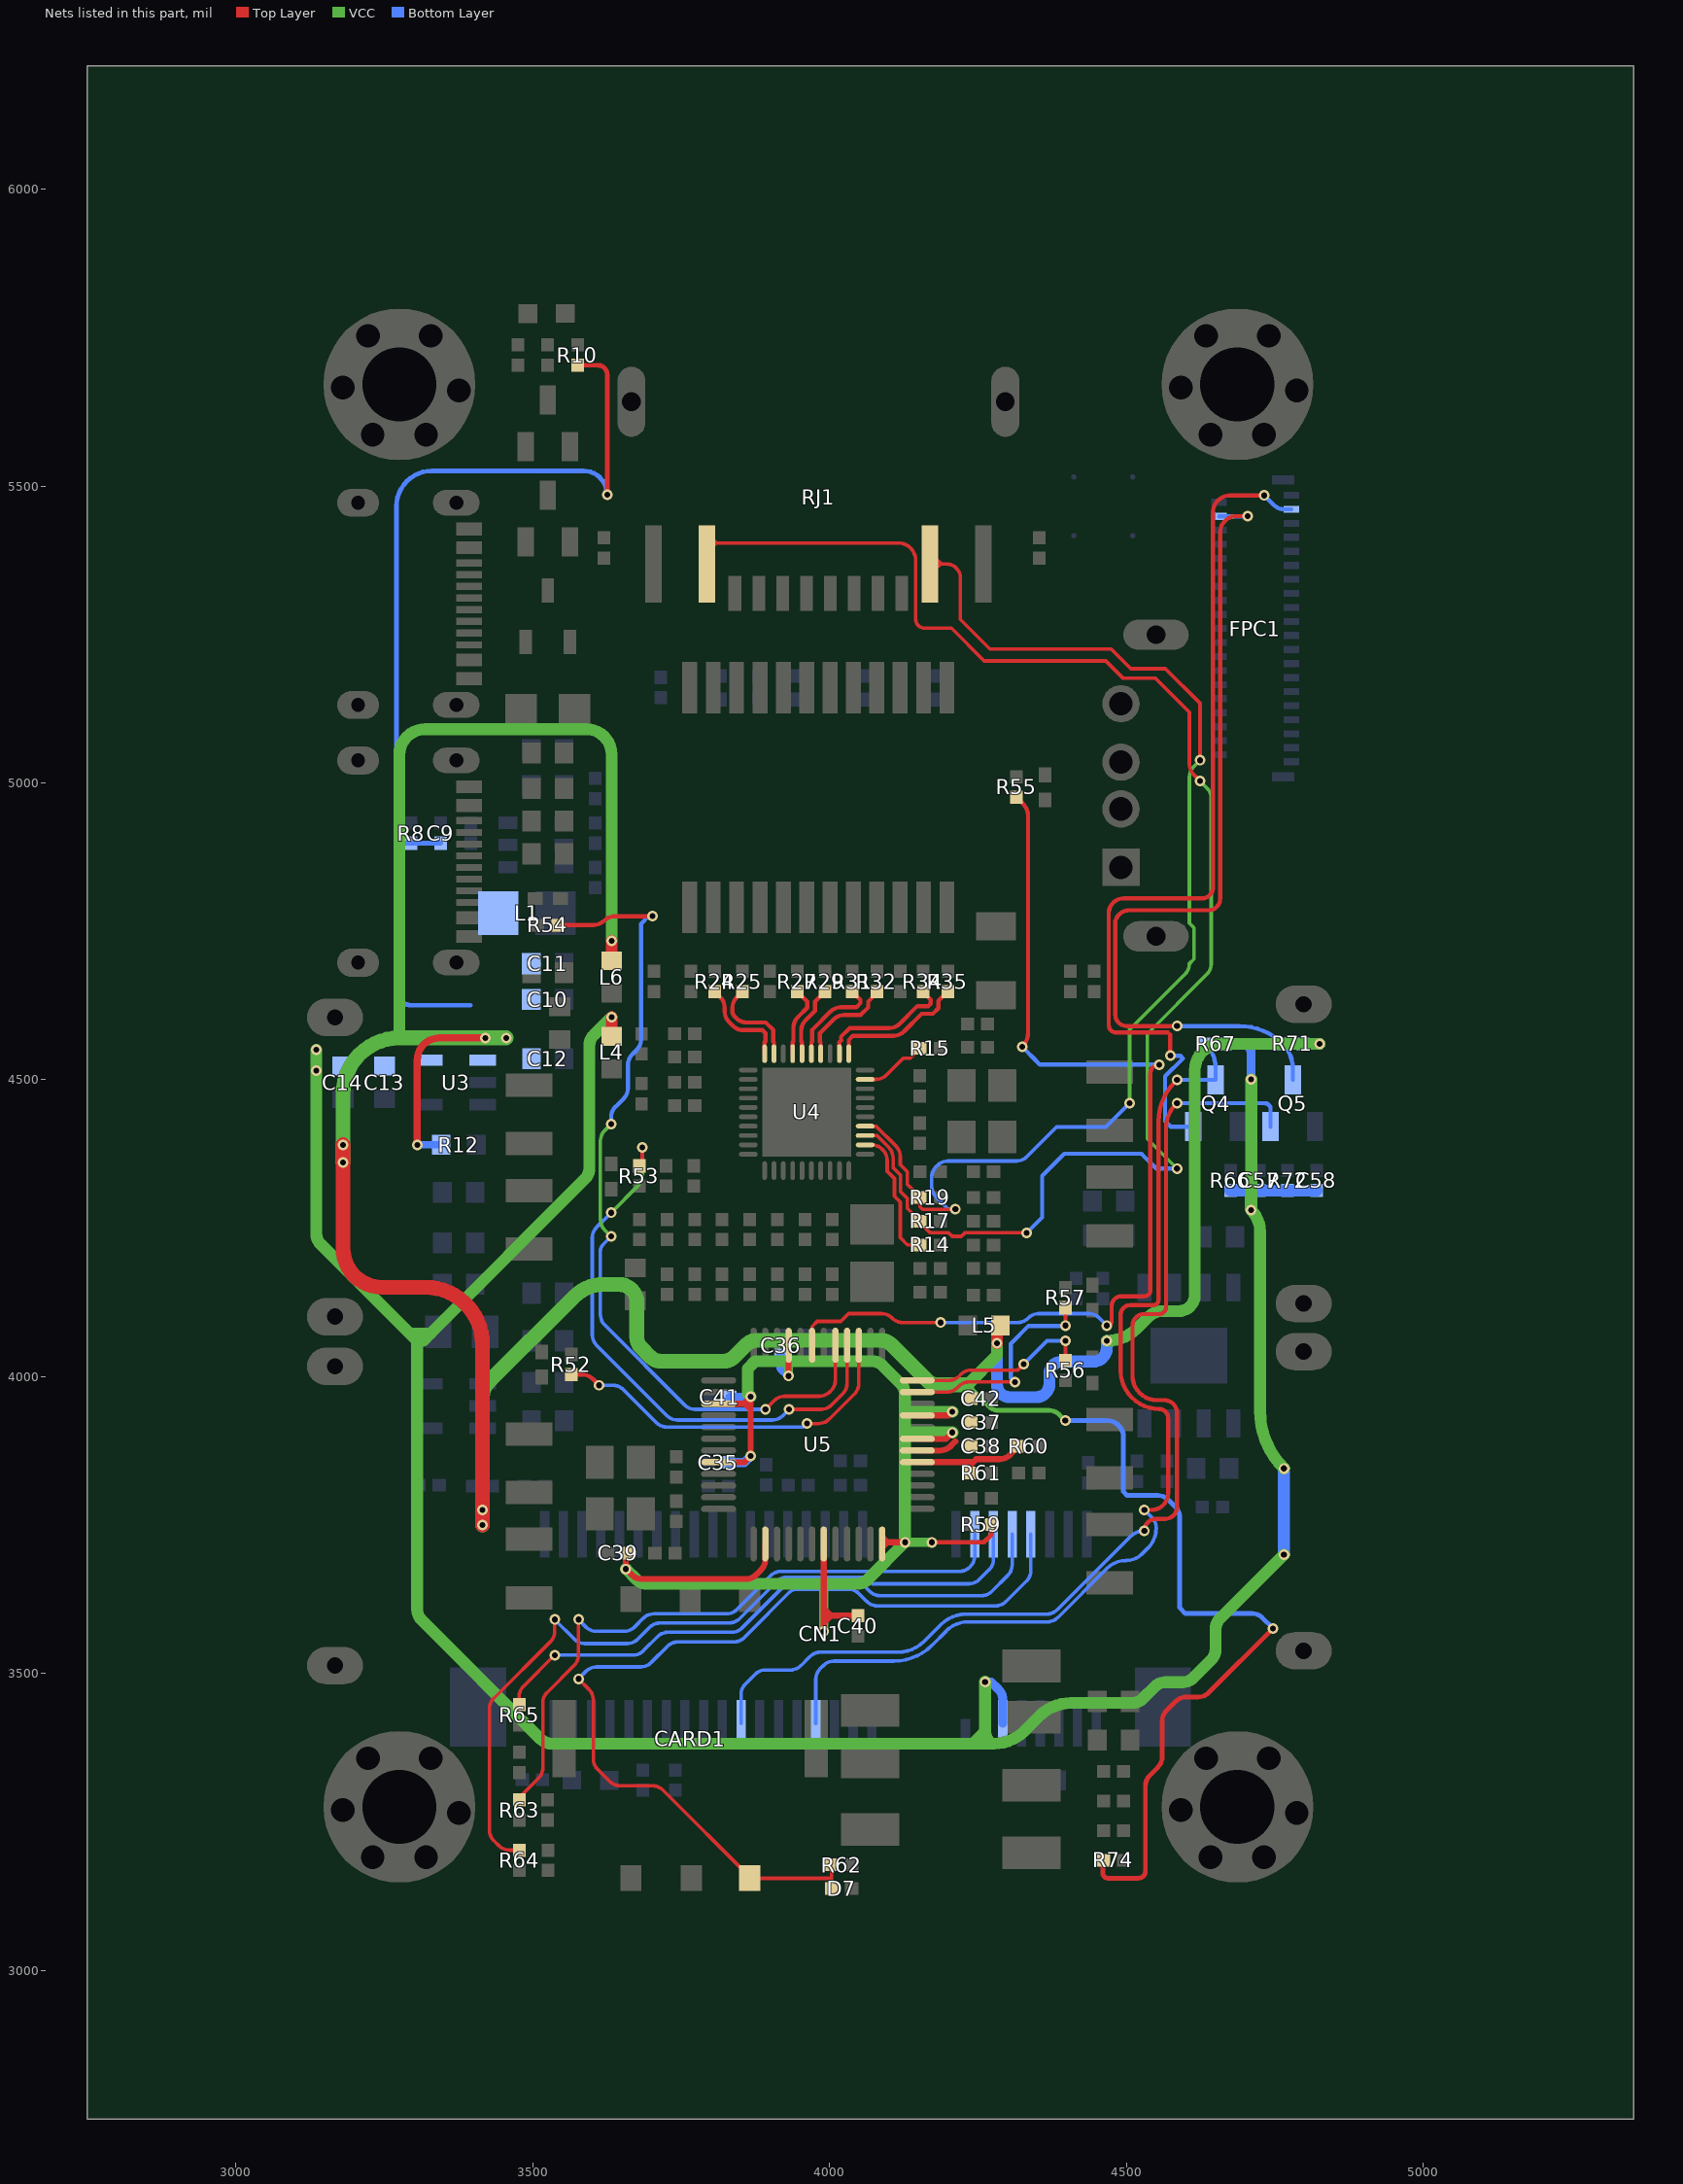
[diagram p0: the nets of this part, all layers, seen from the top]
# Altium PCB MISC84334.PcbDoc (part 7 of 8)
Units mil, origin at the board's own origin, x right, y up, seen from the top; angles counter-clockwise.
Board outline 2605.13 x 3457.4 mil, 4 copper layers (Top Layer, GND, VCC, Bottom Layer), stack 62.447 mil thick; 209 components, 149 nets, 735 pads, 529 vias.

## Via types
v1: diameter 18, hole 10, Top Layer to Bottom Layer, 529 vias

## Nets (pads, with @x,y where several pads share a name; then routed paths per layer and width w, separated by ;. In a path a pad name is that pad's centre, name@x,y a point inside that pad or via, vN(x,y) a via of type N, cw(c..) or ccw(c..) an arc to the next point about the centre after c; other vN are vias at no path point) (continued)
LED1: R52.2 U5.3 | length 616.2
  Top Layer w6: v1(3962.29,3921.19) 3981.94,3921.19 ccw(c3981.94,3946.19) 3999.61,3928.51 4042.17,3971.07 ccw(c4024.49,3988.75) 4049.49,3988.75 U5.3@4049.49,4052.91
  Top Layer w7: R52.2@3565.22,4003.55 3583.98,4003.55 cw(c3583.98,3978.55) 3601.65,3996.23 v1(3612.29,3985.59)
  Bottom Layer w6: v1(3612.29,3985.59) 3635.24,3985.59 cw(c3635.24,3960.59) 3652.91,3978.27 3708.67,3922.51 ccw(c3726.35,3940.19) 3726.35,3915.19 3956.29,3915.19 v1(3962.29,3921.19)
LED2: R53.2 U5.4 | length 966.4
  Top Layer w6: R53.2@3679.83,4355.13 3684.83,4360.13 v1(3684.83,4386.19) ; v1(3932.29,3945.19) 3985.94,3945.19 ccw(c3985.94,3970.19) 4003.61,3952.51 4022.48,3971.38 ccw(c4004.8,3989.06) 4029.8,3989.06 U5.4@4029.8,4052.91
  VCC w6: v1(3632.29,4276.19) 3677.51,4321.41 ccw(c3659.83,4339.09) 3684.83,4339.09 v1(3684.83,4386.19)
  Bottom Layer w6: v1(3632.29,4276.19) 3607.91,4251.81 ccw(c3625.59,4234.14) 3600.59,4234.14 3600.59,4070.52 ccw(c3625.59,4070.52) 3607.91,4052.84 3726.24,3934.51 ccw(c3743.92,3952.19) 3743.92,3927.19 3903.94,3927.19 ccw(c3903.94,3952.19) 3921.61,3934.51 v1(3932.29,3945.19)
LED3: R54.2 U5.5 | length 1428.5
  Top Layer w6: v1(3892.29,3945.19) 3906.98,3959.88 cw(c3924.66,3942.21) 3924.66,3967.21 3982.95,3967.21 ccw(c3982.95,3992.21) 4000.63,3974.53 4002.8,3976.7 ccw(c3985.12,3994.38) 4010.12,3994.38 U5.5@4010.12,4052.91
  Top Layer w7: R54.2@3542.63,4760.59 3602.26,4760.59 ccw(c3602.26,4785.59) 3617.26,4765.59 3623.92,4770.59 cw(c3638.92,4750.59) 3638.92,4775.59 v1@3700.59,4775.59
  VCC w6: v1(3632.29,4236.19) 3621.61,4246.87 cw(c3639.29,4264.55) 3614.29,4264.55 3614.29,4397.24 cw(c3639.29,4397.24) 3621.61,4414.91 v1(3632.29,4425.59)
  Bottom Layer w6: v1(3632.29,4236.19) 3619.12,4223.02 ccw(c3630.8,4211.35) 3614.29,4211.35 3614.29,4104.55 ccw(c3639.29,4104.55) 3621.61,4086.87 3755.97,3952.51 ccw(c3773.65,3970.19) 3773.65,3945.19 v1(3892.29,3945.19)
  Bottom Layer w7: v1(3632.29,4425.59) 3632.29,4436.94 cw(c3657.29,4436.94) 3639.61,4454.61 3653.27,4468.27 ccw(c3635.59,4485.95) 3660.59,4485.95 3660.59,4525.24 cw(c3685.59,4525.24) 3667.91,4542.91 3675.45,4550.45 ccw(c3657.77,4568.12) 3682.77,4568.12 3682.77,4762.77 3695.59,4775.59 v1(3702.29,4775.59)
LED4: R55.2 U5.7 | length 1731.9
  Top Layer w6: U5.7@3970.75,4052.91 3970.75,4084.65 3979.29,4093.19 4019.29,4093.19 4032.29,4106.19 4087.94,4106.19 cw(c4087.94,4081.19) 4105.61,4098.87 4105.97,4098.51 ccw(c4123.65,4116.19) 4123.65,4091.19 v1(4187.29,4091.19)
  Top Layer w7: R55.2@4315.33,4976.05 4325.48,4965.9 cw(c4303.48,4943.91) 4334.59,4943.91 4334.59,4579.25 cw(c4301.13,4579.25) v1(4324.79,4555.59) ; v1(4467.29,4086.19) ccw(c4467.29,4094.49) 4475.59,4094.49 4475.59,4119.14 cw(c4492.04,4119.14) 4492.04,4135.59 4530.59,4135.59 ccw(c4530.59,4145.59) 4540.59,4145.59 4540.59,4510.59 cw(c4555.59,4510.59) v1(4555.59,4525.59)
  Bottom Layer w6: v1(4187.29,4091.19) 4316.94,4091.19 ccw(c4316.94,4116.19) 4334.61,4098.51 4334.97,4098.87 cw(c4352.65,4081.19) 4352.65,4106.19 4436.94,4106.19 cw(c4436.94,4081.19) 4454.61,4098.87 v1(4467.29,4086.19)
  Bottom Layer w7: v1(4324.79,4555.59) 4335.52,4544.86 ccw(c4350.59,4555.59) 4339.86,4540.52 4354.79,4525.59 v1(4555.59,4525.59)
LED5: R56.2 U5.48 | length 308.4
  Top Layer w6: U5.48@4147.91,3993.86 4201.06,3993.86 ccw(c4201.06,4018.86) 4218.74,4001.18 4221.42,4003.86 cw(c4239.1,3986.19) 4239.1,4011.19 4317.29,4011.19 v1(4327.29,4021.19)
  Top Layer w7: R56.2@4397.83,4027.63 v1(4397.83,4060.59)
  Bottom Layer w7: v1(4327.29,4021.19) 4366.69,4060.59 v1(4397.83,4060.59)
LED6: R57.2 U5.47 | length 371.2
  Top Layer w6: U5.47@4147.91,3974.17 4197.64,3974.17 ccw(c4197.64,3999.17) 4215.32,3981.49 4217.69,3983.87 cw(c4235.37,3966.19) 4235.37,3991.19 v1(4312.29,3991.19)
  Top Layer w7: v1(4397.83,4086.19) R57.2@4397.83,4116.05
  Bottom Layer w7: v1(4312.29,3991.19) 4305.59,3997.89 4305.59,4055.59 4335.59,4085.59 4397.23,4085.59 v1(4397.83,4086.19)
MDIN0_PHY: R34.1 U4.2 | length 228.2
  Top Layer w7: U4.2@4016.86,4543.99 4016.86,4563.24 4019.78,4566.16 ; 4019.74,4566.16 4019.74,4572.58 4034.35,4587.19 4100.94,4587.19 ccw(c4100.94,4612.19) 4118.61,4594.51 4148.29,4624.19 4166.64,4624.19 4170.51,4628.05 4170.51,4634.98 4157.86,4647.63 R34.1@4157.86,4648.55
MDIN1_PHY: R31.1 U4.5 | length 164.5
  Top Layer w7: U4.5@3969.66,4543.99 3969.66,4563.24 3971.01,4564.59 3971.01,4584.08 4001.8,4614.87 cw(c4019.48,4597.19) 4019.48,4622.19 4045.29,4622.19 4052.29,4629.19 4052.29,4634.6 4038.75,4648.13 R31.1@4038.75,4648.55
MDIN2_PHY: R27.1 U4.7 | length 120.6
  Top Layer w7: U4.7@3938.16,4543.99 3938.16,4563.24 3939.51,4564.59 3939.51,4588.05 cw(c3964.51,4588.05) 3946.83,4605.73 3962.7,4621.6 3962.7,4631.87 R27.1@3946.02,4648.55
MDIN3_PHY: R24.1 U4.10 | length 162.2
  Top Layer w7: R24.1@3806.91,4648.55 3816.27,4639.19 cw(c3798.6,4621.51) 3823.6,4621.51 3823.6,4615.16 ccw(c3848.6,4615.16) 3830.92,4597.48 3837.39,4591.01 ccw(c3855.07,4608.69) 3855.07,4583.69 3887.26,4583.69 3892.26,4578.69 3892.26,4564.64 3890.86,4563.24 U4.10@3890.86,4543.99
MDIP0_PHY: R35.1 U4.1 | length 229.6
  Top Layer w7: U4.1@4032.66,4543.99 4032.74,4544.07 4032.74,4567.19 4039.74,4574.19 4107.88,4574.19 ccw(c4107.88,4599.19) 4125.56,4581.51 4155.24,4611.19 4174.29,4611.19 4183.79,4620.69 4183.79,4633.12 R35.1@4199.22,4648.55
MDIP1_PHY: R32.1 U4.4 | length 166.1
  Top Layer w7: U4.4@3985.36,4543.99 3985.36,4563.24 3984.01,4564.59 3984.01,4578.69 4007.19,4601.87 cw(c4024.87,4584.19) 4024.87,4609.19 4052.49,4609.19 4065.29,4621.99 4065.29,4631.89 4080.12,4646.72 R32.1@4080.12,4648.55
MDIP2_PHY: R29.1 U4.6 | length 120.6
  Top Layer w7: U4.6@3953.86,4543.99 3953.86,4563.24 3952.51,4564.59 3952.51,4582.67 cw(c3977.51,4582.67) 3959.83,4600.35 3975.7,4616.22 3975.7,4631.87 R29.1@3992.38,4648.55
MDIP3_PHY: R25.1 U4.9 | length 162.6
  Top Layer w7: R25.1@3853.28,4648.55 3843.92,4639.19 ccw(c3861.6,4621.51) 3836.6,4621.51 3836.6,4616.19 ccw(c3851.08,4616.19) 3840.84,4605.95 3842.71,4604.07 ccw(c3860.54,4621.9) 3860.54,4596.69 3892.64,4596.69 3905.26,4584.08 3905.26,4564.64 3906.66,4563.24 U4.9@3906.66,4543.99
PCIE_RX_4G: CN1.23 Q4.3 R67.1 | length 1783.6
  Top Layer w7: v1(4530.59,3775.59) 4542.22,3775.59 ccw(c4542.22,3803.96) 4570.59,3803.96 4570.59,3930.59 ccw(c4555.59,3930.59) 4555.59,3945.59 cw(c4555.59,4010.59) 4490.59,4010.59 4490.59,4104.45 cw(c4506.73,4104.45) 4506.73,4120.59 4545.59,4120.59 ccw(c4545.59,4129.59) 4554.59,4129.59 4554.59,4430.37 cw(c4647.76,4430.37) 4581.88,4496.25 v1(4585.59,4499.96)
  Bottom Layer w6: CN1.23@3977.09,3416.14 3977.09,3490.63 cw(c4002.09,3490.63) 3984.41,3508.31 3989.97,3513.87 cw(c4007.65,3496.19) 4007.65,3521.19 4108.47,3521.19 ccw(c4108.47,3612.25) 4172.86,3547.86 4197.02,3572.02 cw(c4233.65,3535.39) 4233.65,3587.19 4367.02,3587.19 ccw(c4367.02,3612.33) 4384.8,3594.55 4466.86,3676.62 cw(c4500.59,3642.89) 4500.59,3690.59 ccw(c4500.59,3726.8) 4526.2,3701.2 4536.7,3711.7 ccw(c4503.16,3745.24) 4550.59,3745.24 ccw(c4525.59,3745.24) 4543.27,3762.91 v1(4530.59,3775.59)
  Bottom Layer w7: v1(4585.59,4499.96) Q4.3@4650.59,4499.96 4650.59,4519.45 ccw(c4592.41,4519.45) R67.1@4633.55,4560.59
PCIE_TS_RX: FPC1.36 Q5.3 R71.2 | length 1446.6
  Top Layer w7: v1(4585.59,4590.59) 4500.59,4590.59 cw(c4500.59,4609.59) 4481.59,4609.59 4481.59,4767.59 cw(c4505.59,4760.59) 4505.59,4785.59 4638.57,4785.59 ccw(c4638.57,4805.31) 4658.29,4805.31 4658.29,5422.84 cw(c4683.29,5422.84) 4665.61,5440.51 4666.97,5441.87 cw(c4684.65,5424.19) 4684.65,5449.19 v1(4704.29,5449.19)
  Bottom Layer w7: v1(4585.59,4590.59) 4691.12,4590.59 cw(c4691.12,4488.16) R71.2@4763.55,4560.59 cw(c4722.41,4519.45) 4780.59,4519.45 Q5.3@4780.59,4499.96 ; FPC1.36@4656.27,5449.06 4704.16,5449.06 v1(4704.29,5449.19)
PCIE_TS_TX: FPC1.37 Q4.2 | length 1517.4
  Top Layer w7: v1(4574.53,4540.59) 4574.09,4541.03 4574.09,4575.93 4570.43,4579.59 4483.21,4579.59 cw(c4483.21,4592.21) 4470.59,4592.21 4470.59,4780.59 cw(c4495.59,4780.59) 4495.59,4805.59 4627.37,4805.59 ccw(c4627.37,4824.51) 4646.29,4824.51 4646.29,5456.84 cw(c4671.29,5456.84) 4653.61,5474.51 4655.97,5476.87 cw(c4673.65,5459.19) 4673.65,5484.19 v1(4732.29,5484.19)
  Bottom Layer w7: v1(4574.53,4540.59) 4591.12,4540.59 4595.59,4536.12 4565.59,4506.12 4565.59,4430.59 4574.96,4421.22 Q4.2@4613.19,4421.22 ; v1(4732.29,5484.19) 4748.29,5468.19 ccw(c4765.97,5485.87) 4765.97,5460.87 FPC1.37@4778.31,5460.87
PCIE_TX_4G: CN1.31 Q5.2 | length 1883.5
  Top Layer w7: v1(4530.59,3740.59) cw(c4550.59,3740.59) 4550.59,3760.59 4565.59,3760.59 ccw(c4565.59,3780.59) 4585.59,3780.59 4585.59,3939 ccw(c4564,3939) 4564,3960.59 4551.68,3960.59 cw(c4551.68,4001.68) 4510.59,4001.68 4510.59,4086.19 cw(c4529.99,4086.19) 4529.99,4105.59 4555.59,4105.59 ccw(c4555.59,4117.09) 4567.09,4117.09 4567.09,4419.49 cw(c4621.66,4419.49) 4583.07,4458.07 v1(4585.59,4460.59)
  Bottom Layer w6: CN1.31@3851.1,3416.14 3851.1,3464.64 cw(c3876.1,3464.64) 3858.42,3482.32 3874.97,3498.87 cw(c3892.65,3481.19) 3892.65,3506.19 3934.31,3506.19 ccw(c3934.31,3531.19) 3951.98,3513.51 3967.34,3528.87 cw(c3985.02,3511.19) 3985.02,3536.19 4116.08,3536.19 ccw(c4116.08,3596.81) 4158.95,3553.95 4187.19,3582.19 cw(c4230.65,3538.74) 4230.65,3600.19 4365.94,3600.19 ccw(c4365.94,3625.19) 4383.61,3607.51 4506.86,3730.76 cw(c4530.59,3707.03) v1(4530.59,3740.59)
  Bottom Layer w7: v1(4585.59,4460.59) 4733.39,4460.59 cw(c4733.39,4450.79) 4743.19,4450.79 Q5.2@4743.19,4421.22
PHY0_LED0: R14.1 U4.32 | length 229.6
  Top Layer w6: U4.32@4060.16,4390.49 4071.34,4390.49 cw(c4071.34,4365.49) 4089.02,4383.17 4089.97,4382.22 cw(c4072.29,4364.54) 4097.29,4364.54 4097.29,4346.19 4109.61,4333.87 4109.61,4303.87 4119.29,4294.19 4119.29,4234.19 4131.39,4222.09 R14.1@4152.67,4222.09
PHY0_LED1: R17.1 RJ1.10 U4.33 | length 2640.3
  Top Layer w6: RJ1.10@3800.51,5413.32 3809.65,5404.19 ; U4.33@4060.16,4406.19 4080.14,4406.19 4099.97,4386.36 cw(c4082.29,4368.68) 4107.29,4368.68 4107.29,4352.19 4119.85,4339.64 4119.85,4311.64 4131.29,4300.19 4131.29,4283.41 R17.1@4152.61,4262.09 4152.61,4259.48 4167.38,4244.72 ccw(c4173.1,4250.45) 4173.1,4242.35 4201.05,4242.35 4207.05,4236.35 4222.31,4236.35 4228.31,4242.35 v1(4332.29,4242.35) ; v1(4624.29,5003.19) 4613.61,5013.87 cw(c4631.29,5031.55) 4606.29,5031.55 4606.29,5119.16 4549.29,5176.16 4495.02,5176.16 4465.59,5205.59 4260.59,5205.59 4205.59,5260.59 4160.59,5260.59 cw(c4160.59,5275.89) 4145.29,5275.89 4145.29,5374.84 ccw(c4115.94,5374.84) 4115.94,5404.19 3809.77,5404.19 ; 3809.65,5404.19 3809.77,5404.19 ; 3809.65,5404.19 3793.65,5404.19 3793.65,5388.07 3809.77,5404.19
  VCC w6: v1(4585.59,4350.59) 4535.59,4400.59 4535.59,4577.49 4635.97,4677.87 ccw(c4618.29,4695.55) 4643.29,4695.55 4643.29,4973.84 ccw(c4618.29,4973.84) 4635.97,4991.51 v1(4624.29,5003.19)
  Bottom Layer w7: v1(4332.29,4242.35) 4358.29,4268.35 4358.29,4338.29 4395.59,4375.59 4525.59,4375.59 4550.59,4350.59 v1(4585.59,4350.59)
PHY0_LED2: R19.1 RJ1.11 U4.34 | length 2058.9
  Top Layer w6: U4.34@4060.16,4421.99 4078.48,4421.99 4111.97,4388.5 cw(c4094.29,4370.82) 4119.29,4370.82 4119.29,4357.19 4131.36,4345.12 4131.36,4324.12 4152.73,4302.75 R19.1@4152.73,4302.09 4152.73,4286.16 4156.92,4281.98 v1(4212.29,4281.98) ; RJ1.11@4169.24,5368.57 4189.19,5368.57 ; RJ1.11@4179.49,5361.51 4184.69,5366.71 cw(c4189.19,5362.21) 4189.19,5368.57 ; RJ1.11@4179.49,5377.58 4188.02,5369.06 ccw(c4189.19,5370.23) 4189.19,5368.57 ; v1(4624.29,5038.19) 4624.29,5134.19 4566.08,5192.4 4507.66,5192.4 4474.48,5225.59 4270.59,5225.59 4220.59,5275.59 4220.59,5345.59 ccw(c4197.61,5345.59) 4197.61,5368.57 4189.19,5368.57
  VCC w6: v1(4505.59,4460.59) 4505.59,4584.49 4598.97,4677.87 ccw(c4581.29,4695.55) 4606.29,4695.55 4614.24,4703.49 4614.24,4755.98 4606.29,4763.93 4606.29,5009.84 cw(c4631.29,5009.84) 4613.61,5027.51 v1(4624.29,5038.19)
  Bottom Layer w6: v1(4212.29,4281.98) 4200.29,4281.98 4179.61,4302.66 cw(c4197.29,4320.34) 4172.29,4320.34 4172.29,4335.84 cw(c4197.29,4335.84) 4179.61,4353.51 4181.97,4355.87 cw(c4199.65,4338.19) 4199.65,4363.19 4314.94,4363.19 ccw(c4314.94,4388.19) 4332.61,4370.51 4382.69,4420.59 4465.59,4420.59 v1(4505.59,4460.59)
PHY_RSET: R15.1 U4.39 | length 113.4
  Top Layer w6: U4.39@4060.16,4500.69 4078.57,4500.69 ccw(c4078.57,4525.69) 4096.24,4508.01 4124.42,4536.19 4136.29,4536.19 4152.55,4552.45 R15.1@4152.55,4553.09
UIM_CLK: CN1.12 R64.1 | length 1331.5
  Top Layer w6: R64.1@3478.09,3202.63 3461.21,3202.63 cw(c3461.21,3227.63) 3443.53,3209.95 3434.61,3218.87 cw(c3452.29,3236.55) 3427.29,3236.55 3427.29,3440.84 cw(c3452.29,3440.84) 3434.61,3458.51 3529.97,3553.87 ccw(c3512.29,3571.55) 3537.29,3571.55 v1(3537.29,3591.19)
  Bottom Layer w6: v1(3537.29,3591.19) 3570.47,3558.01 ccw(c3588.15,3575.69) 3588.15,3550.69 3659.44,3550.69 ccw(c3659.44,3575.69) 3677.11,3558.01 3697.17,3578.07 cw(c3714.84,3560.39) 3714.84,3585.39 3831.13,3585.39 ccw(c3831.13,3610.39) 3848.81,3592.71 3910.97,3654.87 cw(c3928.65,3637.19) 3928.65,3662.19 4061.29,3662.19 4072.29,3651.19 4234.94,3651.19 ccw(c4234.94,3676.19) 4252.61,3658.51 4268.97,3674.87 ccw(c4251.3,3692.55) 4276.3,3692.55 CN1.12@4276.3,3735.04
UIM_DATA: CN1.10 R65.2 | length 1007.9
  Top Layer w6: R65.2@3478.04,3447.63 3477.29,3448.38 3477.29,3460.84 cw(c3502.29,3460.84) 3484.61,3478.51 v1(3537.29,3531.19)
  Bottom Layer w6: v1(3537.29,3531.19) 3668.94,3531.19 ccw(c3668.94,3556.19) 3686.61,3538.51 3710.41,3562.31 cw(c3728.09,3544.63) 3728.09,3569.63 3835.08,3569.63 ccw(c3835.08,3594.63) 3852.76,3576.96 3920.67,3644.87 cw(c3938.35,3627.19) 3938.35,3652.19 4043.94,3652.19 cw(c4043.94,3627.19) 4061.61,3644.87 4067.97,3638.51 ccw(c4085.65,3656.19) 4085.65,3631.19 4255.94,3631.19 ccw(c4255.94,3656.19) 4273.61,3638.51 4300.46,3665.36 ccw(c4282.79,3683.04) 4307.79,3683.04 CN1.10@4307.79,3735.04
UIM_PWR: CARD1.C1 CN1.8 D7.1 R62.2 | length 1592.2
  Top Layer w6: v1(3577.29,3491.19) 3594.97,3473.51 cw(c3577.29,3455.84) 3602.29,3455.84 3602.29,3356.55 ccw(c3627.29,3356.55) 3609.61,3338.87 3629.97,3318.51 ccw(c3647.65,3336.19) 3647.65,3311.19 3701.94,3311.19 cw(c3701.94,3286.19) 3719.61,3303.87 3865.6,3157.89 CARD1.C1@3865.6,3155.36 4003.69,3155.36 ; D7.1@4003.55,3138.09 ccw(c4003.55,3138.23) 4003.69,3138.23 4003.69,3155.36 ; R62.2@4003.69,3177.96 4003.69,3155.36
  Bottom Layer w6: v1(3577.29,3491.19) 3589.97,3503.87 cw(c3607.65,3486.19) 3607.65,3511.19 3681.94,3511.19 ccw(c3681.94,3536.19) 3699.61,3518.51 3727.21,3546.11 cw(c3744.89,3528.43) 3744.89,3553.43 3839.18,3553.43 ccw(c3839.18,3578.43) 3856.85,3560.75 3897.29,3601.19 3897.29,3601.68 3933.2,3637.59 cw(c3944.31,3626.49) 3944.31,3642.19 4031.94,3642.19 cw(c4031.94,3617.19) 4049.61,3634.87 4062.97,3621.51 ccw(c4080.65,3639.19) 4080.65,3614.19 4279.94,3614.19 ccw(c4279.94,3639.19) 4297.61,3621.51 4331.96,3655.86 ccw(c4314.29,3673.54) 4339.29,3673.54 CN1.8@4339.29,3735.04
UIM_RESET: CN1.14 R63.1 | length 1105.4
  Top Layer w6: R63.1@3477.77,3287.63 3477.77,3291.67 3509.97,3323.87 ccw(c3492.29,3341.55) 3517.29,3341.55 3517.29,3450.84 cw(c3542.29,3450.84) 3524.61,3468.51 3569.97,3513.87 ccw(c3552.29,3531.55) 3577.29,3531.55 v1(3577.29,3591.19)
  Bottom Layer w6: v1(3577.29,3591.19) 3589.97,3578.51 ccw(c3607.65,3596.19) 3607.65,3571.19 3653.94,3571.19 ccw(c3653.94,3596.19) 3671.61,3578.51 3686.45,3593.35 cw(c3704.13,3575.67) 3704.13,3600.67 3826.42,3600.67 ccw(c3826.42,3625.67) 3844.09,3607.99 3900.97,3664.87 cw(c3918.65,3647.19) 3918.65,3672.19 4218.94,3672.19 ccw(c4218.94,3697.19) 4236.61,3679.51 4237.47,3680.37 ccw(c4219.8,3698.05) 4244.8,3698.05 CN1.14@4244.8,3735.04
VBUSM: R60.1 R61.2 U5.41 | length 221.9
  Top Layer w10: U5.41@4147.91,3856.06 4148.04,3856.19 4222.55,3856.19 ; R61.2@4238.56,3838.09 R61.2@4238.56,3840.18 ; R60.1@4318.91,3883.09 4304.33,3868.51 cw(c4286.66,3886.19) 4286.66,3861.19 4247.29,3861.19 4242.29,3856.19 4238.56,3856.19 ; 4222.55,3856.19 R61.2@4238.56,3840.18 ; 4222.55,3856.19 4238.56,3856.19 ; R61.2@4238.56,3840.18 4238.56,3856.19
VCC1V8: C13.2 C14.2 C57.1 C58.2 CN1.11 L4.2 R66.1 R67.2 R72.2 U3.5 | length 4811.7
  Top Layer w20: L4.2@3633.09,4573.41 v1(3633.09,4605.59)
  VCC w20: v1(3135.59,4550.59) v1(3135.59,4515.59) 3135.59,4240.95 ccw(c3160.59,4240.95) 3142.91,4223.27 3293.7,4072.48 ; v1(3633.09,4605.59) 3602.91,4575.41 ccw(c3620.59,4557.74) 3595.59,4557.74 3595.59,4350.95 cw(c3570.59,4350.95) 3588.27,4333.27 3327.48,4072.48 ; v1(4262.29,3486.19) 4262.29,3408.38 ; v1(4710.59,4500.59) v1(4710.59,4280.59) cw(c4674.38,4244.38) 4725.59,4244.38 4725.59,3942.16 ccw(c4862.16,3942.16) v1(4765.59,3845.59) ; v1(4765.59,3700.59) 4657.91,3592.91 ccw(c4675.59,3575.24) 4650.59,3575.24 4650.59,3540.95 cw(c4625.59,3540.95) 4643.27,3523.27 4612.91,3492.91 cw(c4595.24,3510.59) 4595.24,3485.59 4565.95,3485.59 ccw(c4565.95,3460.59) 4548.27,3478.27 4527.91,3457.91 cw(c4510.24,3475.59) 4510.24,3450.59 4406.96,3450.59 ccw(c4406.96,3374.86) 4353.41,3428.41 4328.36,3403.36 cw(c4277.25,3454.47) 4277.25,3382.19 4271.79,3382.19 ; 3293.7,4072.48 3327.48,4072.48 ; 3293.7,4072.48 3305.59,4060.59 ; 3305.59,4060.59 3305.59,3608.25 ccw(c3330.59,3608.25) 3312.91,3590.57 3513.97,3389.51 ccw(c3531.65,3407.19) 3531.65,3382.19 4242.1,3382.19 ; 3305.59,4060.59 3315.59,4060.59 3327.48,4072.48 ; 4242.1,3382.19 4258.05,3398.14 ccw(c4247.82,3408.38) 4262.29,3408.38 ; 4242.1,3382.19 4260.96,3382.19 ; 4260.96,3382.19 4262.29,3383.52 4262.29,3405.13 ; 4260.96,3382.19 4271.79,3382.19 ; 4262.29,3405.13 4262.29,3408.38 ; 4262.29,3405.13 ccw(c4294.73,3405.13) 4271.79,3382.19
  Bottom Layer w15: v1(4262.29,3486.19) 4272.29,3486.19 4284.72,3473.76 cw(c4267.05,3456.08) 4292.05,3456.08 CN1.11@4292.05,3416.14 ; R67.2@4667.63,4560.59 4694.46,4560.59 cw(c4694.46,4544.46) 4710.59,4544.46 v1(4710.59,4500.59)
  Bottom Layer w20: R66.1@4675.59,4313.55 4710.62,4313.55 C57.1@4724.41,4313.55 R72.2@4771.77,4313.55 C58.2@4820.59,4313.55 ; v1(4710.59,4280.59) 4710.59,4313.52 ; v1(4765.59,3700.59) v1(4765.59,3845.59)
VCC3V3_SYS: C9.2 C10.2 C11.2 C12.2 L1.2 L5.2 L6.2 R8.2 R10.2 R12.1 R71.1 R74.2 U3.1 | length 8490.6
  Top Layer w8: R10.2@3575.59,5703.55 3609.61,5703.55 cw(c3609.61,5687.57) 3625.59,5687.57 v1(3625.59,5485.59) ; R74.2@4461.61,3185.59 ccw(c4461.61,3184.57) 4460.59,3184.57 4460.59,3163.91 ccw(c4468.91,3163.91) 4468.91,3155.59 4520.59,3155.59 ccw(c4520.59,3167.29) 4532.29,3167.29 4532.29,3310.84 cw(c4557.29,3310.84) 4539.61,3328.51 4553.27,3342.17 ccw(c4535.59,3359.85) 4560.59,3359.85 4560.59,3420.24 cw(c4585.59,3420.24) 4567.91,3437.91 4583.27,3453.27 cw(c4600.95,3435.59) 4600.95,3460.59 4621.34,3460.59 ccw(c4621.34,3485.59) 4639.01,3467.91 v1(4747.29,3576.19)
  Top Layer w12: v1(3305.59,4390.59) 3305.59,4532.96 cw(c3343.22,4532.96) 3343.22,4570.59 v1(3420.59,4570.59)
  Top Layer w20: L6.2@3633.09,4700.65 v1(3633.09,4734.19) ; v1(4282.29,4056.19) 4282.29,4080.26 L5.2@4288.12,4086.09
  Top Layer w25: v1(3180.59,4390.59) v1(3180.59,4360.59) 3180.59,4216.61 ccw(c3246.61,4216.61) 3246.61,4150.59 3319.51,4150.59 cw(c3319.51,4054.51) 3415.59,4054.51 v1(3415.59,3775.94) v1(3415.59,3750.59)
  VCC w8: 4232.29,3986.19 4267.86,3950.63 ccw(c4285.53,3968.3) 4285.53,3943.3 4369.82,3943.3 cw(c4369.82,3918.3) 4387.5,3935.98 v1(4397.29,3926.19)
  VCC w20: 3275.59,4575.59 3275.59,5046.92 cw(c3319.26,5046.92) 3319.26,5090.59 3590.59,5090.59 cw(c3590.59,5048.09) 3633.09,5048.09 v1(3633.09,4734.19) ; 4232.29,3986.19 4282.29,4036.19 v1(4282.29,4056.19) ; v1(4467.29,4060.59) 4468.01,4060.59 ccw(c4468.01,4130.94) 4517.75,4081.2 4537.64,4101.08 cw(c4560.59,4078.14) 4560.59,4110.59 4588.74,4110.59 ccw(c4588.74,4137.44) 4615.59,4137.44 4615.59,4516.5 cw(c4659.68,4516.5) 4659.68,4560.59 v1(4825.59,4560.59)
  VCC w25: v1(3180.59,4360.59) v1(3180.59,4390.59) 3180.59,4475.59 cw(c3275.59,4475.59) 3275.59,4570.59 v1(3420.59,4570.59) v1(3455.59,4570.59) ; v1(3415.59,3750.59) v1(3415.59,3775.94) 3415.59,3966.45 cw(c3449.73,3966.45) 3425.59,3990.59 3569.38,4134.38 cw(c3620.59,4083.16) 3620.59,4155.59 3645.59,4155.59 cw(c3645.59,4125.59) 3675.59,4125.59 3675.59,4066.55 ccw(c3700.59,4066.55) 3682.91,4048.87 3698.27,4033.51 ccw(c3715.95,4051.19) 3715.95,4026.19 3821.94,4026.19 ccw(c3821.94,4051.19) 3839.61,4033.51 3859.97,4053.87 cw(c3877.65,4036.19) 3877.65,4061.19 4086.94,4061.19 cw(c4086.94,4036.19) 4104.61,4053.87 4164.97,3993.51 ccw(c4182.65,4011.19) 4182.65,3986.19 4232.29,3986.19
  Bottom Layer w8: 3270.59,4909.88 3270.59,4916.82 ; C9.2@3344.86,4898.55 R8.2@3295.59,4898.55 3273.61,4898.55 cw(c3273.61,4901.57) 3270.59,4901.57 ; 3395.59,4625.59 3296.03,4625.59 cw(c3296.03,4651.03) 3270.59,4651.03 3270.59,4901.57 ; v1(3625.59,5485.59) ccw(c3585.59,5485.59) 3585.59,5525.59 3330.59,5525.59 ccw(c3330.59,5465.59) 3270.59,5465.59 3270.59,4916.82 ; v1(4397.29,3926.19) 4468.53,3926.19 cw(c4468.53,3901.19) 4486.21,3918.87 4487.97,3917.11 cw(c4470.29,3899.43) 4495.29,3899.43 4495.29,3806.31 4501.41,3800.19 4552.94,3800.19 cw(c4552.94,3775.19) 4570.61,3792.87 4582.87,3780.61 cw(c4565.19,3762.93) 4590.19,3762.93 4590.19,3610.68 4599.68,3601.19 4711.94,3601.19 cw(c4711.94,3576.19) 4729.61,3593.87 v1(4747.29,3576.19) ; 3270.59,4901.57 3270.59,4916.82
  Bottom Layer w12: v1(3305.59,4390.59) R12.1@3345.93,4390.59
  Bottom Layer w20: v1(4282.29,4056.19) 4282.29,3986.88 ccw(c4303.58,3986.88) 4303.58,3965.59 4348.69,3965.59 ccw(c4348.69,3987.49) 4370.59,3987.49 4370.59,4004.26 cw(c4391.92,4004.26) 4391.92,4025.59 4444.53,4025.59 ccw(c4444.53,4048.35) 4467.29,4048.35 v1(4467.29,4060.59) ; R71.1@4797.63,4560.59 v1(4825.59,4560.59)
VCC3V3_USB: C35.2 C36.2 C37.2 C38.2 C39.2 C40.2 C41.2 C42.2 R59.2 U5.9 U5.15 U5.20 U5.26 U5.31 U5.36 U5.42 U5.43 U5.45 | length 2752.8
  Top Layer w8: v1(4172.29,3721.19) 4260.23,3721.19 4272.64,3733.6 R59.2@4272.64,3751.19
  Top Layer w10: C39.2@3661.23,3703.09 3657.29,3699.15 3657.29,3686.55 ccw(c3682.29,3686.55) 3659.19,3676.98 ccw(c3682.29,3686.55) 3664.61,3668.87 3666.97,3666.51 ccw(c3684.65,3684.19) 3684.65,3659.19 3858.94,3659.19 ccw(c3858.94,3684.19) 3876.61,3666.51 3884.69,3674.59 ccw(c3867.01,3692.27) 3892.01,3692.27 U5.26@3892.01,3718.27 ; U5.20@3813.27,3856.06 3857.16,3856.06 v1(3867.29,3866.19) 3867.29,3944.71 ; U5.15@3813.27,3954.49 3855.59,3954.49 ; U5.9@3931.38,4052.91 v1(3931.38,4001.19) v1@3932.29,4001.19 ; v1(3990.43,3571.19) 3990.43,3585.02 ; U5.31@3990.43,3718.27 3990.43,3610.24 ; C40.2@4048.09,3597.63 4003.05,3597.63 ; U5.36@4088.86,3718.27 4091.78,3721.19 4098.11,3721.19 ; U5.36@4088.91,3706.52 4088.91,3711.99 4098.11,3721.19 ; U5.36@4090.43,3728.87 4098.11,3721.19 ; v1(4127.29,3721.19) 4098.11,3721.19 ; U5.42@4147.91,3875.75 4186.5,3875.75 ccw(c4186.5,3900.75) 4204.17,3883.07 4212.29,3891.19 ; U5.43@4147.91,3895.43 4196.53,3895.43 v1(4207.29,3906.19) ; U5.45@4147.91,3934.8 4200.9,3934.8 v1(4207.29,3941.19) ; 3855.59,3954.49 v1(3867.29,3966.19) 3867.29,3944.71 ; 3855.59,3954.49 3857.51,3954.49 3867.29,3944.71 ; 3990.43,3585.02 4003.05,3597.63 ; 3990.43,3585.02 3990.43,3597.63 ; 3990.43,3597.63 4003.05,3597.63 ; 3990.43,3597.63 3990.43,3610.24 ; 3990.43,3610.24 4003.05,3597.63
  VCC w15: v1(3931.38,4001.19) 3931.38,4025.05 3932.52,4026.19 ; v1(3990.43,3571.19) 3990.43,3650.29 3991.33,3651.19 ; v1(4127.29,3721.19) v1(4172.29,3721.19)
  VCC w20: v1(3657.29,3676.19) 3674.97,3658.51 ccw(c3692.65,3676.19) 3692.65,3651.19 3991.33,3651.19 4046.94,3651.19 ccw(c4046.94,3676.19) 4064.61,3658.51 v1(4127.29,3721.19) 4127.29,3909.66 ; v1(3867.29,3966.19) 3862.29,3971.19 3862.29,4013.59 3874.89,4026.19 3932.52,4026.19 4071.94,4026.19 cw(c4071.94,4001.19) 4089.61,4018.87 4119.97,3988.51 cw(c4102.29,3970.84) 4127.29,3970.84 4127.29,3909.66 ; 4132.29,3941.19 v1(4207.29,3941.19) ; v1(4207.29,3906.19) 4130.76,3906.19 4127.29,3909.66
  Bottom Layer w15: C35.2@3830.13,3855.59 3856.69,3855.59 v1(3867.29,3866.19) ; C41.2@3832.63,3965.59 3866.69,3965.59 v1(3867.29,3966.19) ; C36.2@3918.09,4036.05 3918.09,4014.48 v1(3931.38,4001.19)